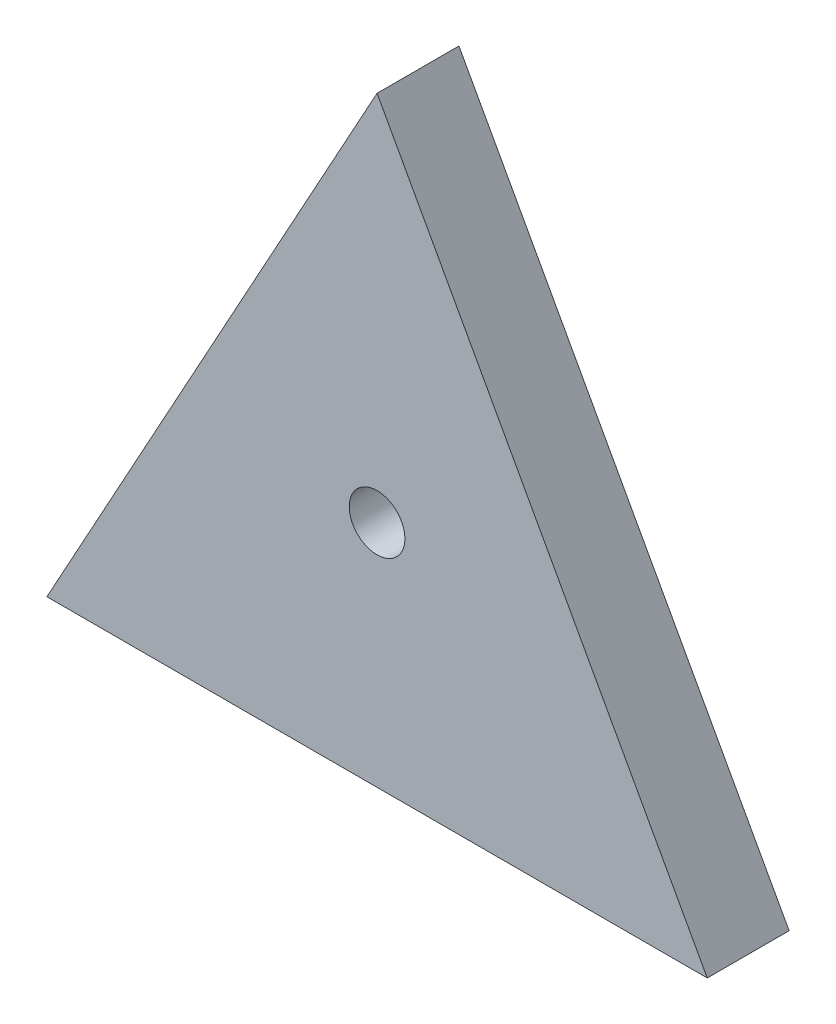
SolidWorks part; units mm, degrees
material "1023 碳钢板 (SS)"
ref_plane "Front Plane" through (0, 0, 0) normal (0, 0, 1) x (1, 0, 0)
ref_plane "Top Plane" through (0, 0, 0) normal (0, 1, 0) x (1, 0, 0)
ref_plane "Right Plane" through (0, 0, 0) normal (1, 0, 0) x (0, 0, -1)
sketch "Sketch1" plane through (0, 0, 0) normal (0, 0, 1) x (1, 0, 0)
  line L0 (0, 0) -> (-60.5, -110.1401)
  line L1 (-60.5, -110.1401) -> (60.5, -110.1401)
  line L2 (60.5, -110.1401) -> (0, 0)
  circle A0 centre (0, -68.1401) radius 4.5
  dimension "D3" = 42
  dimension "D4" = 9
  dimension "D1" = 57.56
  dimension "D2" = 121
extrude "Boss-Extrude1" add sketch "Sketch1" along normal blind 15
hole_wizard "M12 Tapped Hole1" positions "Sketch2" profile "Sketch3" tap size "M12" standard "ISO"
sketch "Sketch2" plane through (0, 0, 15) normal (0, 0, 1) x (1, 0, 0)
  point P0 (0, -68.1401)
sketch "Sketch3" plane through (0, -68.1401, 15) normal (1, 0, 0) x (0, -1, 0)
  line L0 (0, 0) -> (0, 32.3144)
  line L1 (0, 32.3144) -> (5.1, 29.25)
  line L2 (5.1, 29.25) -> (5.1, 0)
  line L5 (5.1, 0) -> (0, 0)
  line L10 (0, 32.3144) -> (-5.1, 29.25) construction
  line L11 (0, -6.35) -> (0, 107.95) construction
  dimension "螺纹孔钻头直径" = 10.2
  dimension "螺纹孔钻头深度" = 29.25
  dimension "导头角度" = 118
cosmetic thread "Hole Thread Line 1" parameters "D1"=24, "D2"=12
